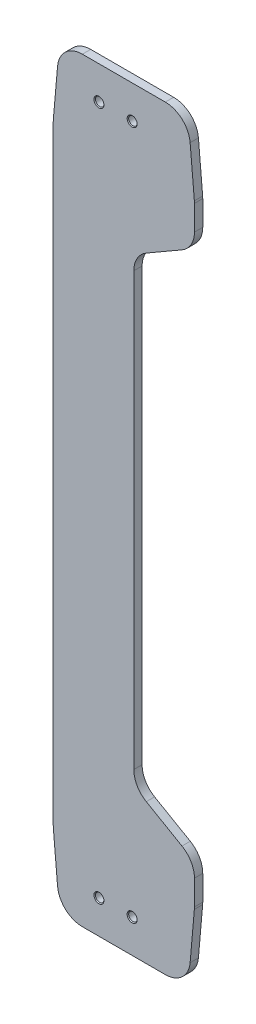
SolidWorks part; units mm, degrees
material "Q345 "
ref_plane "前视基准面" through (0, 0, 0) normal (0, 0, 1) x (1, 0, 0)
ref_plane "上视基准面" through (0, 0, 0) normal (0, 1, 0) x (1, 0, 0)
ref_plane "右视基准面" through (0, 0, 0) normal (1, 0, 0) x (0, 0, -1)
sketch "草图1" plane through (0, 0, 0) normal (0, 0, 1) x (1, 0, 0)
  line L0 (-84.8019, -1426.5116) -> (-89.8858, -1368.4023)
  line L1 (-90, -1365.7876) -> (-90, -632.2124)
  line L2 (-54.9161, -1453.8969) -> (44.9161, -1453.8969)
  line L3 (-5, -1453.8969) -> (-5, -1243.0354) construction
  line L4 (74.8019, -1426.5116) -> (79.8858, -1368.4023)
  line L5 (-125, -2215) -> (-125, 0) construction
  line L6 (80, -1365.7876) -> (80, -1335.7876)
  line L7 (65, -1309.8068) -> (22, -1284.9808)
  line L8 (7, -1259) -> (7, -739)
  line L9 (7, -999) -> (-31.2944, -999) construction
  line L10 (37, -999) -> (7, -999) construction
  line L12 (37, -770.0276) -> (37, -1227.9724) construction
  line L13 (-5, -544.1031) -> (-5, -754.9646) construction
  line L14 (65, -688.1932) -> (22, -713.0192)
  line L15 (80, -632.2124) -> (80, -662.2124)
  line L16 (74.8019, -571.4884) -> (79.8858, -629.5977)
  line L17 (-54.9161, -544.1031) -> (44.9161, -544.1031)
  line L18 (-84.8019, -571.4884) -> (-89.8858, -629.5977)
  line L20 (111, -1253.8969) -> (57, -1253.8969) construction
  arc A0 (22, -1284.9808) -> (7, -1259) centre (37, -1259) cw
  arc A1 (-89.8858, -629.5977) -> (-90, -632.2124) centre (-60, -632.2124) ccw
  arc A2 (-54.9161, -544.1031) -> (-84.8019, -571.4884) centre (-54.9161, -574.1031) ccw
  arc A3 (74.8019, -571.4884) -> (44.9161, -544.1031) centre (44.9161, -574.1031) ccw
  arc A4 (79.8858, -629.5977) -> (80, -632.2124) centre (50, -632.2124) cw
  arc A5 (80, -662.2124) -> (65, -688.1932) centre (50, -662.2124) cw
  arc A6 (22, -713.0192) -> (7, -739) centre (37, -739) ccw
  arc A7 (65, -1309.8068) -> (80, -1335.7876) centre (50, -1335.7876) cw
  arc A8 (80, -1365.7876) -> (79.8858, -1368.4023) centre (50, -1365.7876) cw
  arc A9 (74.8019, -1426.5116) -> (44.9161, -1453.8969) centre (44.9161, -1423.8969) cw
  arc A10 (-84.8019, -1426.5116) -> (-54.9161, -1453.8969) centre (-54.9161, -1423.8969) ccw
  arc A11 (-90, -1365.7876) -> (-89.8858, -1368.4023) centre (-60, -1365.7876) ccw
  point P23 (7, -1276.3205)
  point P27 (-82.406, -544.1031)
  point P30 (72.406, -544.1031)
  point P33 (80, -630.9026)
  point P36 (80, -679.5329)
  point P39 (7, -721.6795)
  point P42 (80, -1318.4671)
  point P45 (80, -1367.0974)
  point P48 (72.406, -1453.8969)
  point P51 (-82.406, -1453.8969)
  point P54 (-90, -1367.0974)
  dimension "D3" = 30
  dimension "D1" = 120
  dimension "D2" = 35
  dimension "D4" = 30
  dimension "D5" = 200
  dimension "D6" = 175
  dimension "D7" = 120
  dimension "D8" = 30
  dimension "D9" = 520
  dimension "D10" = 175
extrude "凸台-拉伸1" add sketch "草图1" along normal blind 10
sketch "草图6" plane through (0, 0, 10) normal (0, 0, 1) x (1, 0, 0)
  line L0 (-35, -584.1031) -> (5, -584.1031) construction
  line L1 (-90, -999) -> (7, -999) construction
  line L2 (-90, -632.2124) -> (-90, -1365.7876) construction
  line L3 (7, -1259) -> (7, -739) construction
  line L4 (44.9161, -544.1031) -> (-54.9161, -544.1031) construction
  circle A0 centre (5, -584.1031) radius 6
  circle A1 centre (-35, -584.1031) radius 6
  circle A2 centre (-35, -1413.8969) radius 6
  circle A3 centre (5, -1413.8969) radius 6
  dimension "D1" = 12
  dimension "D2" = 40
  dimension "D3" = 40
  dimension "D4" = 55
hole_wizard "M12 螺纹孔1" positions "3D草图1" profile "草图7" tap size "M12" standard "GB" end condition through all
sketch3d "3D草图1"
  point P0 (5, -1413.8969, 10)
  point P3 (-35, -1413.8969, 10)
  point P6 (-35, -584.1031, 10)
  point P9 (5, -584.1031, 10)
sketch "草图7" plane through (5, -1413.8969, 10) normal (1, 0, 0) x (0, -1, 0)
  line L0 (0, 0) -> (0, 10)
  line L1 (0, 10) -> (5.1, 10)
  line L2 (5.1, 10) -> (5.1, 0.925)
  line L3 (5.1, 0.925) -> (6.025, 0)
  line L5 (6.025, 0) -> (0, 0)
  line L6 (-5.1, 0.925) -> (-6.025, 0) construction
  line L11 (0, -6.35) -> (0, 107.95) construction
  dimension "通孔螺纹孔钻头直径" = 10.2
  dimension "通孔螺纹孔钻头深度" = 10
  dimension "近端锥形沉头孔直径" = 12.05
  dimension "近端锥形沉头孔角度" = 90
cosmetic thread "孔螺蚊线1" parameters "D2"=12
cosmetic thread "孔螺蚊线2" parameters "D2"=12
cosmetic thread "孔螺蚊线3" parameters "D2"=12
cosmetic thread "孔螺蚊线4" parameters "D2"=12
